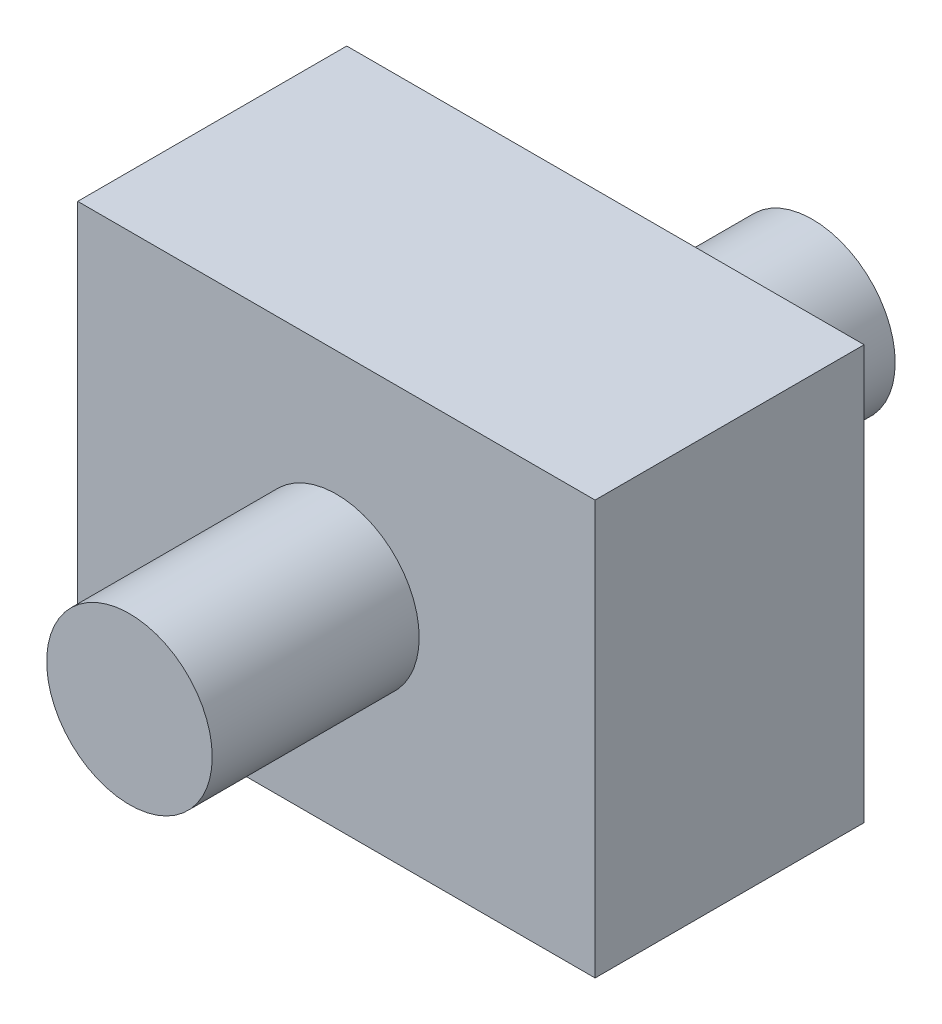
from build123d import *

# Parameters (mm, degrees)
SKETCH1_W           = 25
SKETCH1_H           = 13
BOSS_EXTRUDE1_DEPTH = 20
SKETCH2_R           = 4
BOSS_EXTRUDE2_DEPTH = 10


with BuildPart() as part:
    # Sketch1 → Boss-Extrude1 (new body)
    with BuildSketch(Plane(origin=(0, 0, 0), x_dir=(1, 0, 0), z_dir=(0, 1, 0))):
        Rectangle(SKETCH1_W, SKETCH1_H)
    extrude(amount=BOSS_EXTRUDE1_DEPTH)

    # Sketch2 → Boss-Extrude2 (add)
    with BuildSketch(Plane.XY.offset(6.5)):
        with Locations((0, 10)):
            Circle(SKETCH2_R)
    boss_extrude2 = extrude(amount=BOSS_EXTRUDE2_DEPTH)

    # Mirror1: Boss-Extrude2 across plane
    add(boss_extrude2.mirror(Plane.XY))


solid = part.part
